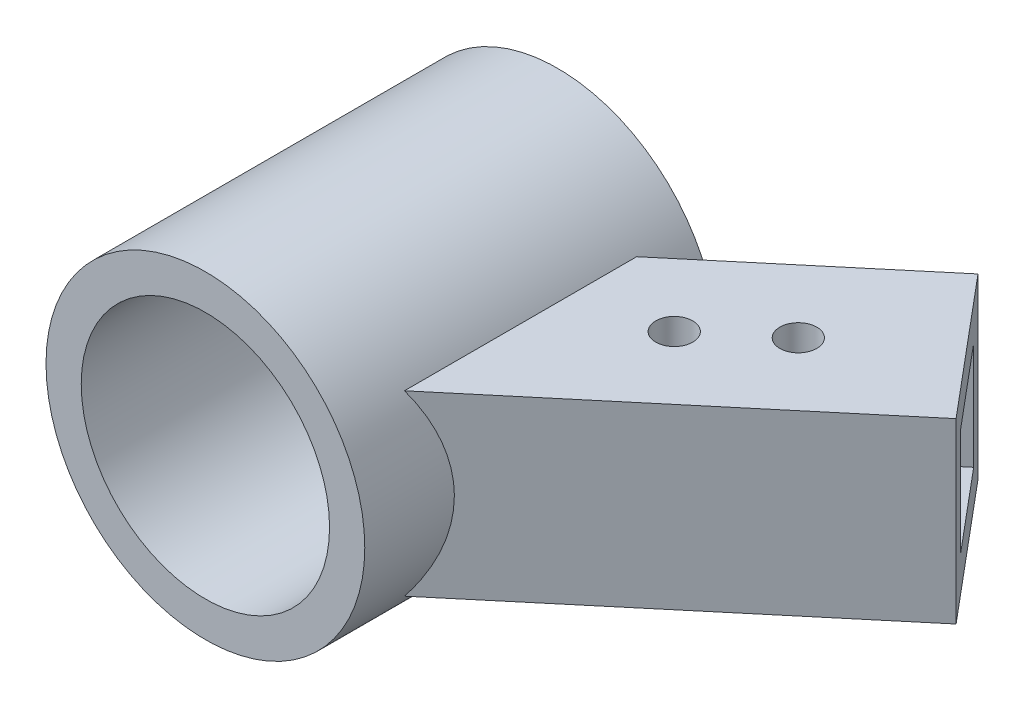
from build123d import *

# Parameters (mm, degrees)
SKETCH_1_R          = 45.25
SKETCH_1_R_2        = 35.25
EXTRUDE_1_DEPTH     = 50
EXTRUDE_2_DEPTH     = 15.25
EXTRUDE_3_DEPTH     = 10
SKETCH_5_R          = 5.25
CUT_EXTRUDE_1_DEPTH = 82.5


with BuildPart() as part:
    # 草图1 → 凸台-拉伸1 (new, symmetric)
    with BuildSketch(Plane.XY):
        Circle(SKETCH_1_R)
        Circle(SKETCH_1_R_2, mode=Mode.SUBTRACT)
    extrude(amount=EXTRUDE_1_DEPTH, both=True)

    # 草图2 → 凸台-拉伸2 (add, symmetric)
    with BuildSketch(Plane(origin=(0, 0, 0), x_dir=(1, 0, 0), z_dir=(0, 1, 0))):
        Polygon((90.237954411, 79.101906321), (35.25, 32.961534056), (35.25, 19.907461162), (96.665830508, 71.44146189), align=None)
        Polygon((122.6987287, 40.416661944), (116.270852604, 48.077106375), (35.25, -19.907461162), (35.25, -32.961534056), align=None)
    extrude(amount=EXTRUDE_2_DEPTH, both=True)

    # 草图4 → 凸台-拉伸3 (add)
    with BuildSketch(Plane(origin=(0, 15.25, 0), x_dir=(1, 0, 0), z_dir=(0, 1, 0))):
        Polygon((90.237954411, 79.101906321), (122.6987287, 40.416661944), (35.25, -32.961534056), (35.25, 32.961534056), align=None)
    extrude_3 = extrude(amount=EXTRUDE_3_DEPTH)

    # 镜向1: 凸台-拉伸3 across plane
    add(extrude_3.mirror(Plane.ZX))

    # 草图5 → 切除-拉伸1 (cut, symmetric)
    with BuildSketch(Plane(origin=(0, 25.25, 0), x_dir=(1, 0, 0), z_dir=(0, 1, 0))):
        with Locations(Location((80.42283049, 37.904505403, 0), (0, 0, 270))):
            Circle(SKETCH_5_R)
        with Locations(Location((61.271719412, 21.834815161, 0), (0, 0, 270))):
            Circle(SKETCH_5_R)
    extrude(amount=CUT_EXTRUDE_1_DEPTH, both=True, mode=Mode.SUBTRACT)


solid = part.part
